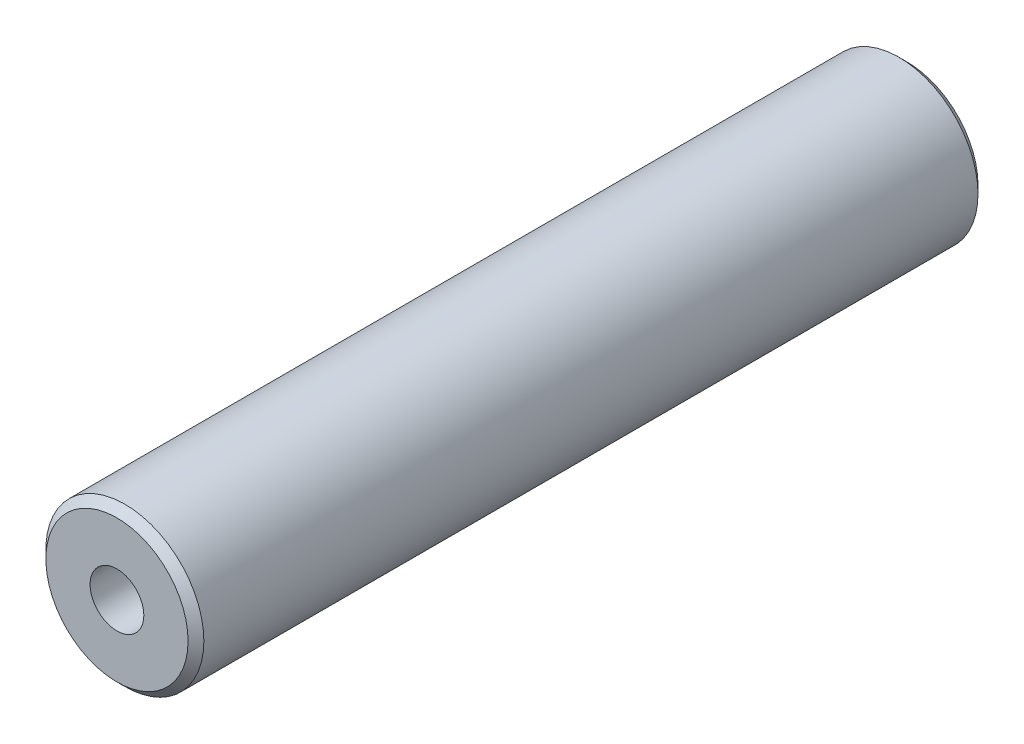
from build123d import *

# Parameters (mm, degrees)
SKETCH1_R             = 10
BOSS_EXTRUDE1_DEPTH   = 100
M8_TAPPED_HOLE1_D     = 6.8
M8_TAPPED_HOLE1_DEPTH = 22.25
M8_TAPPED_HOLE1_TIP   = 2.042926105
CHAMFER1_SIZE         = 1
CHAMFER3_SIZE         = 1
M8_TAPPED_HOLE2_D     = 6.8
M8_TAPPED_HOLE2_DEPTH = 22.25
M8_TAPPED_HOLE2_TIP   = 2.042926105


with BuildPart() as part:
    # Sketch1 → Boss-Extrude1 (new body)
    with BuildSketch(Plane.XY):
        Circle(SKETCH1_R)
    extrude(amount=BOSS_EXTRUDE1_DEPTH)

    # M8 Tapped Hole1
    with Locations(Plane.XY.offset(100)):
        with Locations((0, 0)):
            Hole(M8_TAPPED_HOLE1_D / 2, depth=M8_TAPPED_HOLE1_DEPTH)
            with Locations((0, 0, -(M8_TAPPED_HOLE1_DEPTH + M8_TAPPED_HOLE1_TIP / 2))):  # 118° drill point
                Cone(0, M8_TAPPED_HOLE1_D / 2, M8_TAPPED_HOLE1_TIP, mode=Mode.SUBTRACT)

    # Chamfer1
    chamfer1_edges = [part.edges().sort_by_distance(p)[0] for p in [
        (-10, 0, 100),
    ]]
    chamfer(chamfer1_edges, length=CHAMFER1_SIZE)

    # Chamfer3
    chamfer3_edges = [part.edges().sort_by_distance(p)[0] for p in [
        (-10, 0, 0),
    ]]
    chamfer(chamfer3_edges, length=CHAMFER3_SIZE)

    # M8 Tapped Hole2
    with Locations(Plane(origin=(0, 0, 0), x_dir=(-1, 0, 0), z_dir=(0, 0, -1))):
        with Locations((0, 0)):
            Hole(M8_TAPPED_HOLE2_D / 2, depth=M8_TAPPED_HOLE2_DEPTH)
            with Locations((0, 0, -(M8_TAPPED_HOLE2_DEPTH + M8_TAPPED_HOLE2_TIP / 2))):  # 118° drill point
                Cone(0, M8_TAPPED_HOLE2_D / 2, M8_TAPPED_HOLE2_TIP, mode=Mode.SUBTRACT)


solid = part.part
